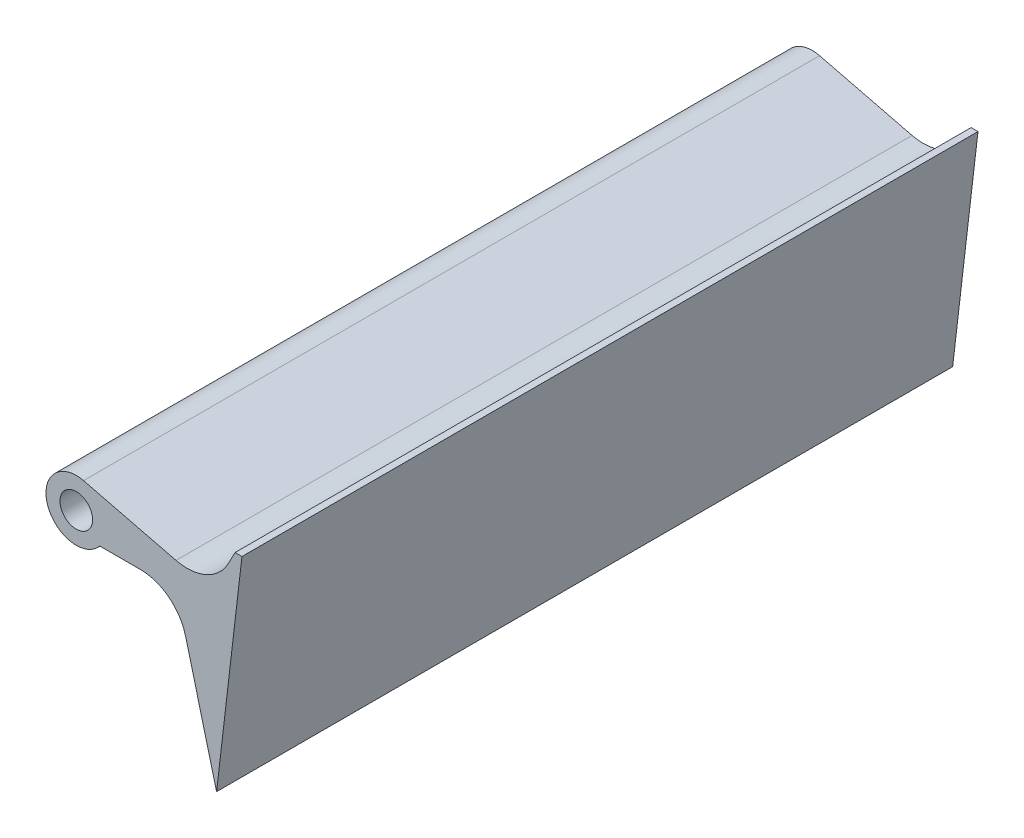
from build123d import *

# Parameters (mm, degrees)
SKETCH1_R           = 17.5
BOSS_EXTRUDE1_DEPTH = 790
FILLET1_R           = 50
FILLET3_R           = 50


with BuildPart() as part:
    # Sketch1 → Boss-Extrude1 (new body)
    with BuildSketch(Plane.XY):
        with BuildLine():
            Line((7.791320793, 31.552263315), (145.258384303, -2.393003291))
            Line((145.258384303, -2.393003291), (170.412288606, 46.028262492))
            Line((170.412288606, 46.028262492), (177.818310073, 46.028262492))
            Line((177.818310073, 46.028262492), (150.622769958, -186.130384226))
            Line((150.622769958, -186.130384226), (107.433938335, -20.538722405))
            Line((107.433938335, -20.538722405), (25.187514406, -20.538722405))
            ThreePointArc((25.187514406, -20.538722405), (-30.82642683, -10.294727238), (7.791320793, 31.552263315))
        make_face()
        with Locations(Location((0, 0, 0), (0, 0, 180))):
            Circle(SKETCH1_R, mode=Mode.SUBTRACT)
    extrude(amount=BOSS_EXTRUDE1_DEPTH)

    # Fillet1
    fillet1_edges = [part.edges().sort_by_distance(p)[0] for p in [
        (145.258384303, -2.393003291, 395),
    ]]
    fillet(fillet1_edges, radius=FILLET1_R)

    # Fillet3
    fillet3_edges = [part.edges().sort_by_distance(p)[0] for p in [
        (107.433938335, -20.538722405, 395),
    ]]
    fillet(fillet3_edges, radius=FILLET3_R)


solid = part.part
